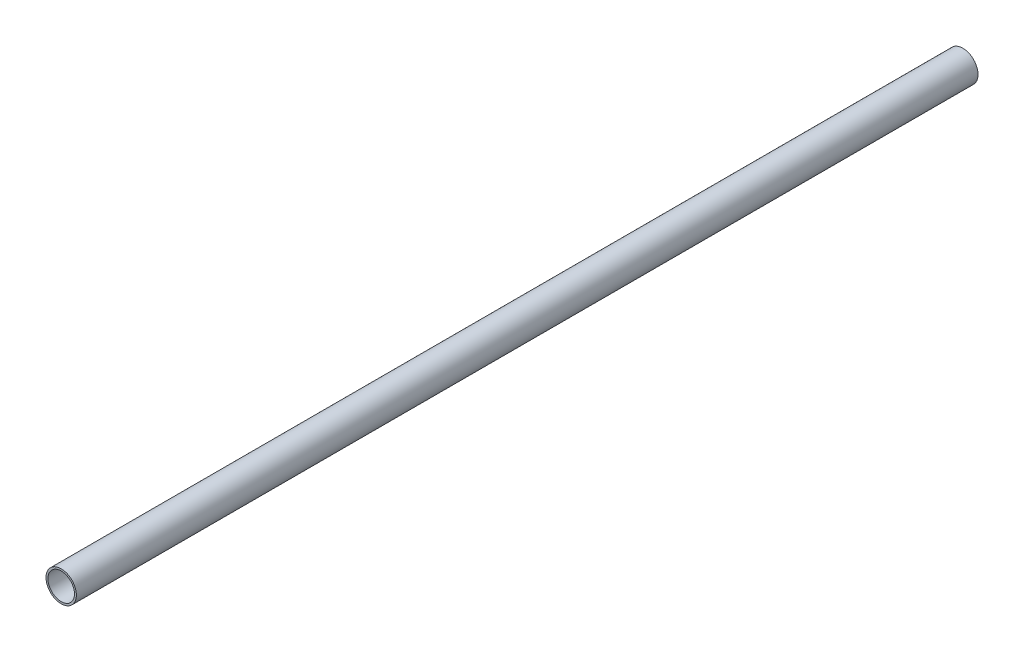
SolidWorks part; units mm, degrees
ref_plane "前视基准面" through (0, 0, 0) normal (0, 0, 1) x (1, 0, 0)
ref_plane "上视基准面" through (0, 0, 0) normal (0, 1, 0) x (1, 0, 0)
ref_plane "右视基准面" through (0, 0, 0) normal (1, 0, 0) x (0, 0, -1)
sketch "草图1" plane through (0, 0, 0) normal (0, 0, 1) x (1, 0, 0)
  circle A0 centre (0, 0) radius 16
  circle A1 centre (0, 0) radius 14
  dimension "D1" = 32
  dimension "D2" = 2
extrude "凸台-拉伸1" add sketch "草图1" along normal mid plane 950
